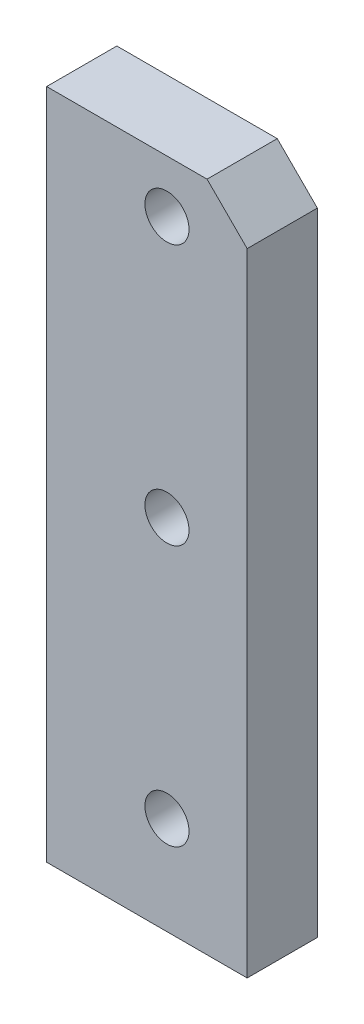
SolidWorks part; units mm, degrees
ref_plane "前视基准面" through (0, 0, 0) normal (0, 0, 1) x (1, 0, 0)
ref_plane "上视基准面" through (0, 0, 0) normal (0, 1, 0) x (1, 0, 0)
ref_plane "右视基准面" through (0, 0, 0) normal (1, 0, 0) x (0, 0, -1)
sketch "草图1" plane through (0, 0, 0) normal (0, 0, 1) x (1, 0, 0)
  line L1 (50, 167.5) -> (-50, 167.5)
  line L2 (50, 167.5) -> (50, -167.5)
  line L3 (50, -167.5) -> (-50, -167.5)
  line L4 (-50, 167.5) -> (-50, -167.5)
  line L5 (50, 167.5) -> (-50, -167.5) construction
  line L6 (50, -167.5) -> (-50, 167.5) construction
  point P0 (0, 0)
  dimension "D1" = 100
  dimension "D2" = 335
extrude "凸台-拉伸1" add sketch "草图1" along normal blind 35
chamfer "倒角1" distance 20 angle 45 1 edges at (50, 167.5, 17.5)
sketch "草图2" plane through (0, 0, 35) normal (0, 0, 1) x (1, 0, 0)
  line L0 (10, 167.5) -> (10, -182.5) construction
  line L1 (30, 167.5) -> (-50, 167.5) construction
  line L3 (50, -167.5) -> (50, 147.5) construction
  circle A0 centre (10, 141.3276) radius 11
  circle A1 centre (10, -118.6724) radius 11
  circle A2 centre (10, 11.3276) radius 11
  dimension "D1" = 22
  dimension "D2" = 40
  dimension "D4" = 130
  dimension "D3" = 260
extrude "切除-拉伸1" cut sketch "草图2" against normal through all both and the other way through all
